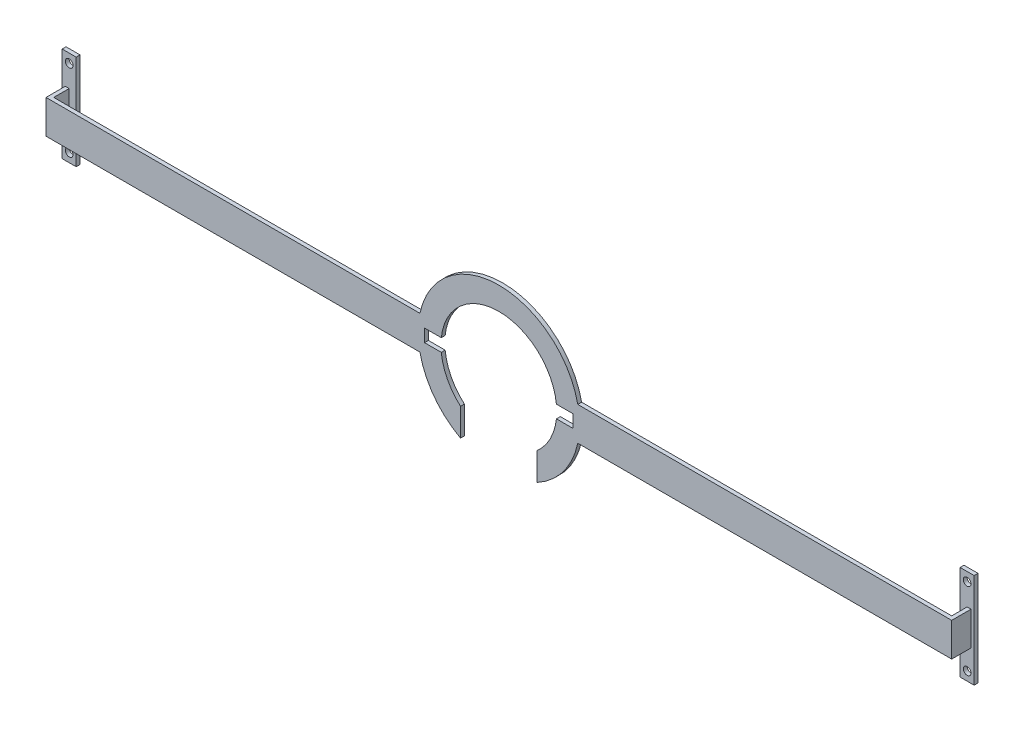
from build123d import *

# Parameters (mm, degrees)
BOSS_EXTRUDE1_DEPTH = 1
SKETCH2_W           = 1
SKETCH2_H           = 8.697838108
BOSS_EXTRUDE2_DEPTH = 6
SKETCH3_W           = 3.625858974
SKETCH3_H           = 24.597729298
SKETCH3_R           = 1
BOSS_EXTRUDE3_DEPTH = 1


with BuildPart() as part:
    # Sketch1 → Boss-Extrude1 (new body)
    with BuildSketch(Plane.XY):
        with BuildLine():
            Line((117.275298476, 4.348919054), (20.445206114, 4.348919054))
            ThreePointArc((20.445206114, 4.348919054), (0, 20.902620649), (-20.445206114, 4.348919054))
            Line((-20.445206114, 4.348919054), (-117.275298476, 4.348919054))
            Line((-117.275298476, 4.348919054), (-117.275298476, -4.348919054))
            Line((-117.275298476, -4.348919054), (-20.445206114, -4.348919054))
            ThreePointArc((-20.445206114, -4.348919054), (-16.73157253, -12.528927754), (-9.927442271, -18.394712283))
            Line((-9.927442271, -18.394712283), (-9.927442271, -11.244816137))
            ThreePointArc((-9.927442271, -11.244816137), (-13.314654662, -6.907964333), (-14.909922164, -1.641408252))
            Line((-14.909922164, -1.641408252), (-19.244314933, -1.641408252))
            Line((-19.244314933, -1.641408252), (-19.244314933, 1.641408252))
            Line((-19.244314933, 1.641408252), (-14.909922164, 1.641408252))
            ThreePointArc((-14.909922164, 1.641408252), (0, 15), (14.909922164, 1.641408252))
            Line((14.909922164, 1.641408252), (19.244314933, 1.641408252))
            Line((19.244314933, 1.641408252), (19.244314933, -1.641408252))
            Line((19.244314933, -1.641408252), (14.909922164, -1.641408252))
            ThreePointArc((14.909922164, -1.641408252), (13.314654662, -6.907964333), (9.927442271, -11.244816137))
            Line((9.927442271, -11.244816137), (9.927442271, -18.394712283))
            ThreePointArc((9.927442271, -18.394712283), (16.73157253, -12.528927754), (20.445206114, -4.348919054))
            Line((20.445206114, -4.348919054), (117.275298476, -4.348919054))
            Line((117.275298476, -4.348919054), (117.275298476, 4.348919054))
        make_face()
    extrude(amount=-BOSS_EXTRUDE1_DEPTH)

    # Sketch2 → Boss-Extrude2 (add)
    with BuildSketch(Plane.XY):
        with Locations((-116.775298476, 0)):
            Rectangle(SKETCH2_W, SKETCH2_H)
        with Locations((116.775298476, 0)):
            Rectangle(SKETCH2_W, SKETCH2_H)
    extrude(amount=-BOSS_EXTRUDE2_DEPTH)

    # Sketch3 → Boss-Extrude3 (add)
    # profile 1 of 2: a face of its own
    with BuildSketch(Plane.XY.offset(-6)):
        with Locations((-116.275298476, 0)):
            Rectangle(SKETCH3_W, SKETCH3_H)
        with Locations((-116.275298476, -10)):
            Circle(SKETCH3_R, mode=Mode.SUBTRACT)
        with Locations((-116.275298476, 10)):
            Circle(SKETCH3_R, mode=Mode.SUBTRACT)
    # profile 2 of 2: a face of its own
    with BuildSketch(Plane.XY.offset(-6)):
        with Locations((116.275298476, 0)):
            Rectangle(SKETCH3_W, SKETCH3_H)
        with Locations(Location((116.275298476, 10, 0), (0, 0, 180))):
            Circle(SKETCH3_R, mode=Mode.SUBTRACT)
        with Locations(Location((116.275298476, -10, 0), (0, 0, 180))):
            Circle(SKETCH3_R, mode=Mode.SUBTRACT)
    extrude(amount=BOSS_EXTRUDE3_DEPTH)


solid = part.part
